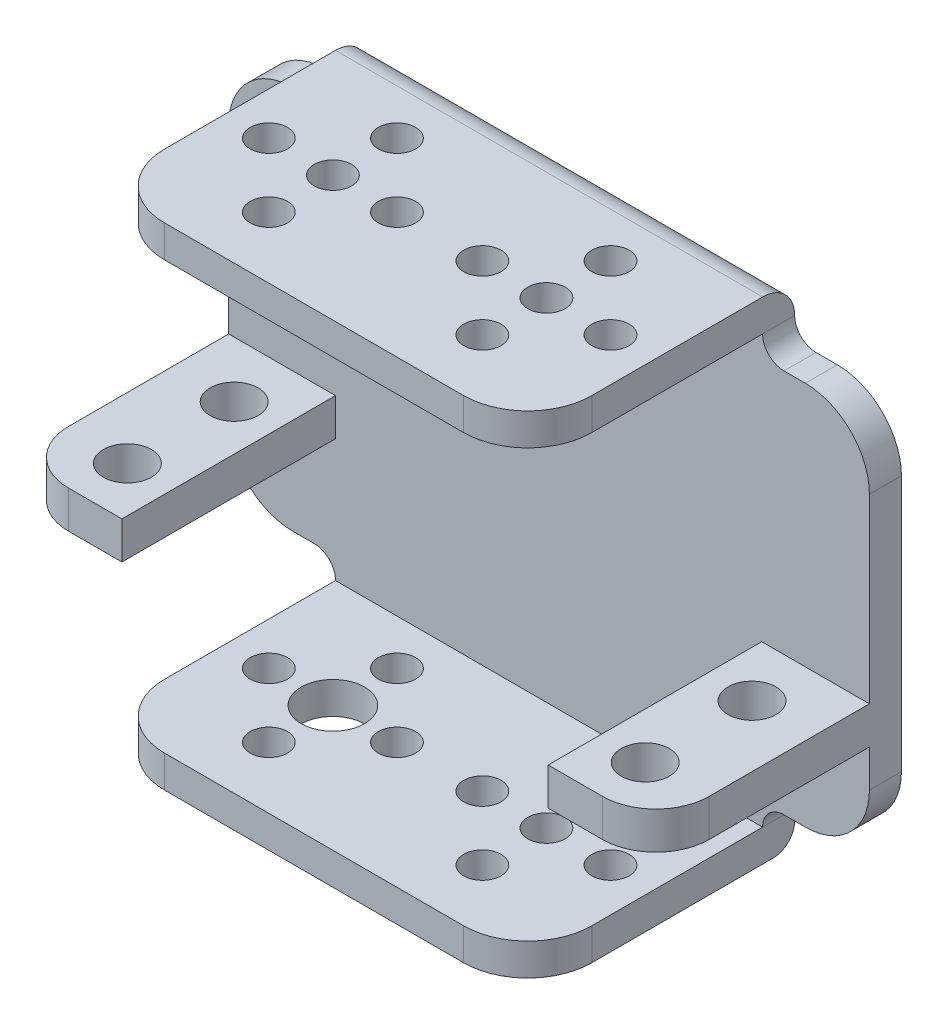
from build123d import *

# Parameters (mm, degrees)
SKETCH1_W           = 60
SKETCH1_H           = 36
BOSS_EXTRUDE1_DEPTH = 3
BOSS_EXTRUDE2_DEPTH = 20
FILLET2_R           = 3
FILLET3_R           = 2
FILLET4_R           = 2
FILLET5_R           = 2
FILLET6_R           = 6
FILLET7_R           = 6
SKETCH4_R           = 1.75
CUT_EXTRUDE1_DEPTH  = 64.238774978
SKETCH6_W           = 10.083484861
SKETCH6_H           = 3.5
SKETCH6_W_2         = 10
BOSS_EXTRUDE3_DEPTH = 20
FILLET8_R           = 5
SKETCH7_R           = 2.25
CUT_EXTRUDE2_DEPTH  = 54.622687928
SKETCH8_R           = 2.97
CUT_EXTRUDE3_DEPTH  = 20
SKETCH9_R           = 1.75
CUT_EXTRUDE4_DEPTH  = 64.238774978
SKETCH10_R          = 1.75
CUT_EXTRUDE5_DEPTH  = 20


with BuildPart() as part:
    # Sketch1 → Boss-Extrude1 (new body)
    with BuildSketch(Plane.XY):
        with Locations((5.470306746, 1.845866319)):
            Rectangle(SKETCH1_W, SKETCH1_H)
    extrude(amount=BOSS_EXTRUDE1_DEPTH)

    # Sketch3 → Boss-Extrude2 (add, symmetric)
    with BuildSketch(Plane(origin=(5.470306746, 0, 0), x_dir=(0, 0, -1), z_dir=(1, 0, 0))):
        Polygon((0, 22.869721484), (0, 24.845866319), (-25, 24.845866319), (-25, 21.845866319), (-3, 21.845866319), (-3, 19.845866319), (0, 19.845866319), align=None)
    boss_extrude2 = extrude(amount=BOSS_EXTRUDE2_DEPTH, both=True)

    # Fillet2
    fillet2_edges = [part.edges().sort_by_distance(p)[0] for p in [
        (5.470306746, 24.845866319, 0),
    ]]
    fillet(fillet2_edges, radius=FILLET2_R)

    # Fillet3
    fillet3_edges = [part.edges().sort_by_distance(p)[0] for p in [
        (-14.529693254, 19.845866319, 1.5),
        (25.470306746, 19.845866319, 1.5),
    ]]
    fillet(fillet3_edges, radius=FILLET3_R)

    # Mirror2: Boss-Extrude2 across plane
    add(boss_extrude2.mirror(Plane(origin=(0, 1.845866319, 0), x_dir=(0, 0, 1), z_dir=(0, -1, 0))))

    # Fillet4
    fillet4_edges = [part.edges().sort_by_distance(p)[0] for p in [
        (25.470306746, -16.154133681, 1.5),
        (-14.529693254, -16.154133681, 1.5),
    ]]
    fillet(fillet4_edges, radius=FILLET4_R)

    # Fillet5
    fillet5_edges = [part.edges().sort_by_distance(p)[0] for p in [
        (5.470306746, -21.154133681, 0),
    ]]
    fillet(fillet5_edges, radius=FILLET5_R)

    # Fillet6
    fillet6_edges = [part.edges().sort_by_distance(p)[0] for p in [
        (-24.529693254, -16.154133681, 1.5),
        (-24.529693254, 19.845866319, 1.5),
        (35.470306746, -16.154133681, 1.5),
        (35.470306746, 19.845866319, 1.5),
    ]]
    fillet(fillet6_edges, radius=FILLET6_R)

    # Fillet7
    fillet7_edges = [part.edges().sort_by_distance(p)[0] for p in [
        (-14.529693254, 23.345866319, 25),
        (25.470306746, 23.345866319, 25),
        (25.470306746, -19.654133681, 25),
        (-14.529693254, -19.654133681, 25),
    ]]
    fillet(fillet7_edges, radius=FILLET7_R)

    # Sketch4 → Cut-Extrude1 (cut, through all)
    with BuildSketch(Plane(origin=(0, 24.845866319, 0), x_dir=(1, 0, 0), z_dir=(0, 1, 0))):
        with Locations(Location((15.423860137, -19.2, 0), (0, 0, 270))):
            Circle(SKETCH4_R)
        with Locations(Location((9.423860137, -13.2, 0), (0, 0, 270))):
            Circle(SKETCH4_R)
        with Locations(Location((15.423860137, -7.2, 0), (0, 0, 270))):
            Circle(SKETCH4_R)
        with Locations(Location((21.423860137, -13.2, 0), (0, 0, 270))):
            Circle(SKETCH4_R)
        with Locations(Location((15.423860137, -13.2, 0), (0, 0, 270))):
            Circle(SKETCH4_R)
    extrude(amount=-CUT_EXTRUDE1_DEPTH, mode=Mode.SUBTRACT)

    # Sketch6 → Boss-Extrude3 (add)
    with BuildSketch(Plane.XY.offset(3)):
        with Locations((30.428564316, -4.904133681)):
            Rectangle(SKETCH6_W, SKETCH6_H)
        with Locations((-19.529693254, -4.904133681)):
            Rectangle(SKETCH6_W_2, SKETCH6_H)
    extrude(amount=BOSS_EXTRUDE3_DEPTH)

    # Fillet8
    fillet8_edges = [part.edges().sort_by_distance(p)[0] for p in [
        (35.470306746, -4.904133681, 23),
        (-24.529693254, -4.904133681, 23),
    ]]
    fillet(fillet8_edges, radius=FILLET8_R)

    # Sketch7 → Cut-Extrude2 (cut, through all)
    with BuildSketch(Plane.XZ.offset(6.654133681)):
        with Locations(Location((29.720306746, 18.243434955, 0), (0, 0, 270))):
            Circle(SKETCH7_R)
        with Locations(Location((29.720306746, 8.243434955, 0), (0, 0, 270))):
            Circle(SKETCH7_R)
        with Locations(Location((-18.779693254, 18.243434955, 0), (0, 0, 270))):
            Circle(SKETCH7_R)
        with Locations(Location((-18.779693254, 8.243434955, 0), (0, 0, 270))):
            Circle(SKETCH7_R)
    extrude(amount=-CUT_EXTRUDE2_DEPTH, mode=Mode.SUBTRACT)

    # Sketch8 → Cut-Extrude3 (cut)
    with BuildSketch(Plane.XZ.offset(21.154133681)):
        with Locations(Location((-4.529693254, 13.243434955, 0), (0, 0, 270))):
            Circle(SKETCH8_R)
    extrude(amount=-CUT_EXTRUDE3_DEPTH, mode=Mode.SUBTRACT)

    # Sketch9 → Cut-Extrude4 (cut, through all)
    with BuildSketch(Plane.XZ.offset(21.154133681)):
        with Locations(Location((-4.529693254, 19.243434955, 0), (0, 0, 270))):
            Circle(SKETCH9_R)
        with Locations(Location((1.470306746, 13.243434955, 0), (0, 0, 270))):
            Circle(SKETCH9_R)
        with Locations(Location((-4.529693254, 7.243434955, 0), (0, 0, 270))):
            Circle(SKETCH9_R)
        with Locations(Location((-10.529693254, 13.243434955, 0), (0, 0, 270))):
            Circle(SKETCH9_R)
    extrude(amount=-CUT_EXTRUDE4_DEPTH, mode=Mode.SUBTRACT)

    # Sketch10 → Cut-Extrude5 (cut)
    with BuildSketch(Plane(origin=(0, 24.845866319, 0), x_dir=(1, 0, 0), z_dir=(0, 1, 0))):
        with Locations(Location((-4.529693254, -13.243434955, 0), (0, 0, 270))):
            Circle(SKETCH10_R)
    extrude(amount=-CUT_EXTRUDE5_DEPTH, mode=Mode.SUBTRACT)


solid = part.part
